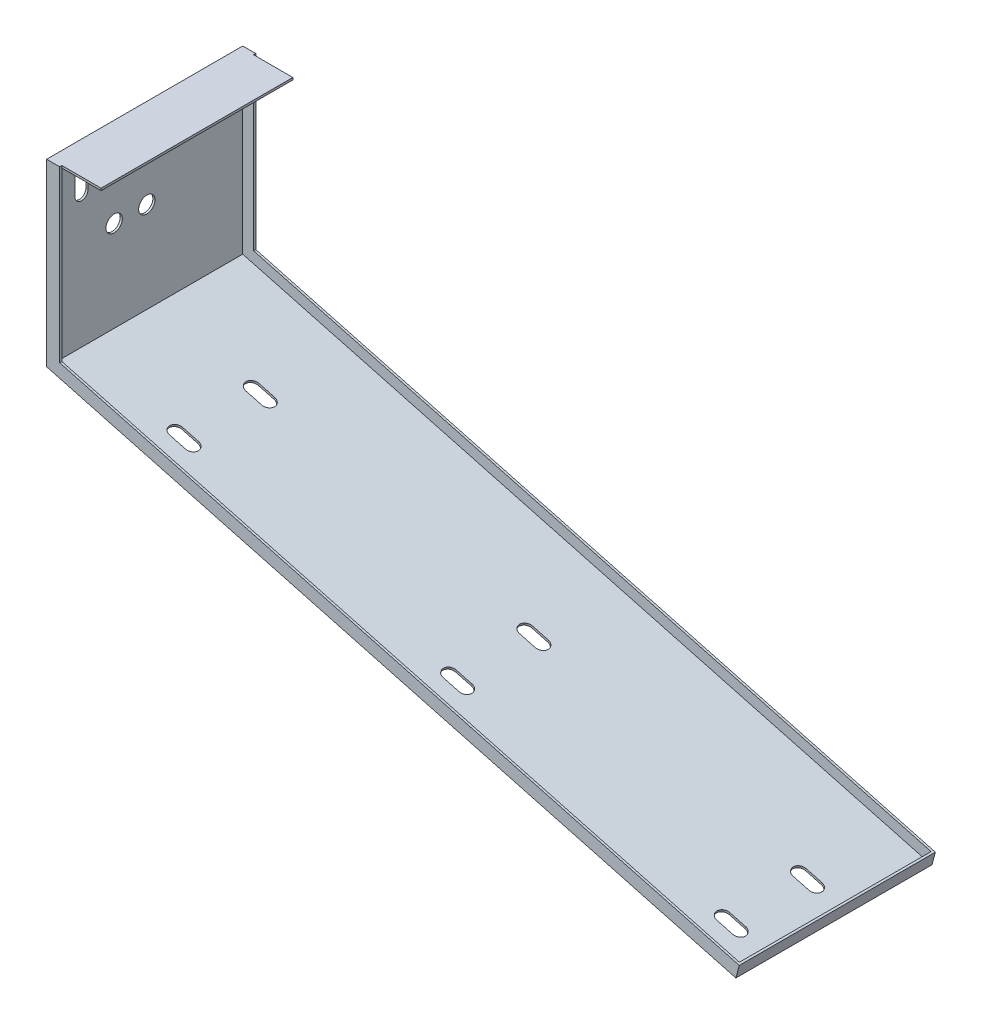
SolidWorks part; units mm, degrees
material "Plain Carbon Steel"
ref_plane "Front Plane" through (0, 0, 0) normal (0, 0, 1) x (1, 0, 0)
ref_plane "Top Plane" through (0, 0, 0) normal (0, 1, 0) x (1, 0, 0)
ref_plane "Right Plane" through (0, 0, 0) normal (1, 0, 0) x (0, 0, -1)
sketch "Sketch1" plane through (0, 0, 0) normal (0, 0, 1) x (1, 0, 0)
  line L0 (0, 0) -> (0, 165)
  line L1 (0, 0) -> (632.6814, -169.5265)
  line L2 (0, 165) -> (48, 165)
  dimension "D1" = 165
  dimension "D2" = 655
  dimension "D3" = 105
  dimension "D4" = 48
extrude "Extrude-Thin1" add sketch "Sketch1" along normal blind 176 thin
sketch "Sketch2" plane through (0, 0, 176) normal (0, 0, 1) x (1, 0, 0)
  line L0 (0, 165) -> (0, 0)
  line L1 (0, 0) -> (632.6814, -169.5265)
  line L2 (632.6814, -169.5265) -> (0, 0) construction
extrude "Extrude-Thin2" add sketch "Sketch2" along normal blind 2 thin thin type one direction reverse wall 12
sketch "Sketch3" plane through (0, 0, 0) normal (0, 0, -1) x (-1, 0, 0)
  line L0 (0, 165) -> (0, 0)
  line L1 (0, 0) -> (-632.6814, -169.5265)
extrude "Extrude-Thin3" add sketch "Sketch3" along normal blind 2 thin
sketch "Sketch4" plane through (0.5176, 1.9319, 0) normal (0.2588, 0.9659, 0) x (0.9659, -0.2588, 0)
  line L1 (655, 0) -> (1.5347, 0) construction
  line L2 (655, -176) -> (653, -176)
  line L3 (655, -176) -> (655, 0)
  line L4 (655, 0) -> (653, 0)
  line L5 (653, -176) -> (653, 0)
  dimension "D1" = 2
extrude "Boss-Extrude1" add sketch "Sketch4" along normal blind 10
sketch "Sketch5" plane through (0, 0, 0) normal (-0.2588, -0.9659, 0) x (0.9659, -0.2588, 0)
  line L0 (611.5, 148) -> (626.5, 148) construction
  line L1 (611.5, 154) -> (626.5, 154)
  line L2 (611.5, 142) -> (626.5, 142)
  line L4 (655, 178) -> (655, -2) construction
  line L5 (0, 178) -> (655, 178) construction
  arc A0 (611.5, 154) -> (611.5, 142) centre (611.5, 148) ccw
  arc A1 (626.5, 142) -> (626.5, 154) centre (626.5, 148) ccw
  point P2 (619, 148)
  dimension "D4" = 6
  dimension "D1" = 30
  dimension "D2" = 36
  dimension "D3" = 15
extrude "Cut-Extrude1" cut sketch "Sketch5" against normal blind 2
sketch "Sketch6" plane through (2, 0, 0) normal (1, 0, 0) x (0, 0, -1)
  line L0 (-148, 139.0347) -> (-148, 124.0347) construction
  line L1 (-142, 139.0347) -> (-142, 124.0347)
  line L2 (-154, 139.0347) -> (-154, 124.0347)
  line L3 (-176, 1.5347) -> (0, 1.5347) construction
  line L5 (-178, 165) -> (-178, 0) construction
  arc A0 (-142, 139.0347) -> (-154, 139.0347) centre (-148, 139.0347) ccw
  arc A1 (-154, 124.0347) -> (-142, 124.0347) centre (-148, 124.0347) ccw
  point P2 (-148, 131.5347)
  dimension "D4" = 6
  dimension "D1" = 130
  dimension "D2" = 30
  dimension "D3" = 15
extrude "Cut-Extrude2" cut sketch "Sketch6" against normal blind 2
sketch "Sketch7" plane through (0, 0, 0) normal (-1, 0, 0) x (0, 0, 1)
  line L0 (-2, 165) -> (-2, 0) construction
  line L1 (178, 0) -> (-2, 0) construction
  circle A0 centre (88, 85) radius 7.5
  dimension "D3" = 15
  dimension "D1" = 90
  dimension "D2" = 85
extrude "Cut-Extrude3" cut sketch "Sketch7" against normal blind 2
pattern_linear "LPattern3" count 2 spacing 30 along (0, 0, 1) of "Cut-Extrude3"
pattern_linear "LPattern4" count 2 spacing 70 along (0, 0, -1) count 3 spacing 260 along (-0.9659, 0.2588, 0) of "Cut-Extrude1"
pattern_linear "LPattern5" count 2 spacing 70 along (0, 0, -1) of "Cut-Extrude2"
